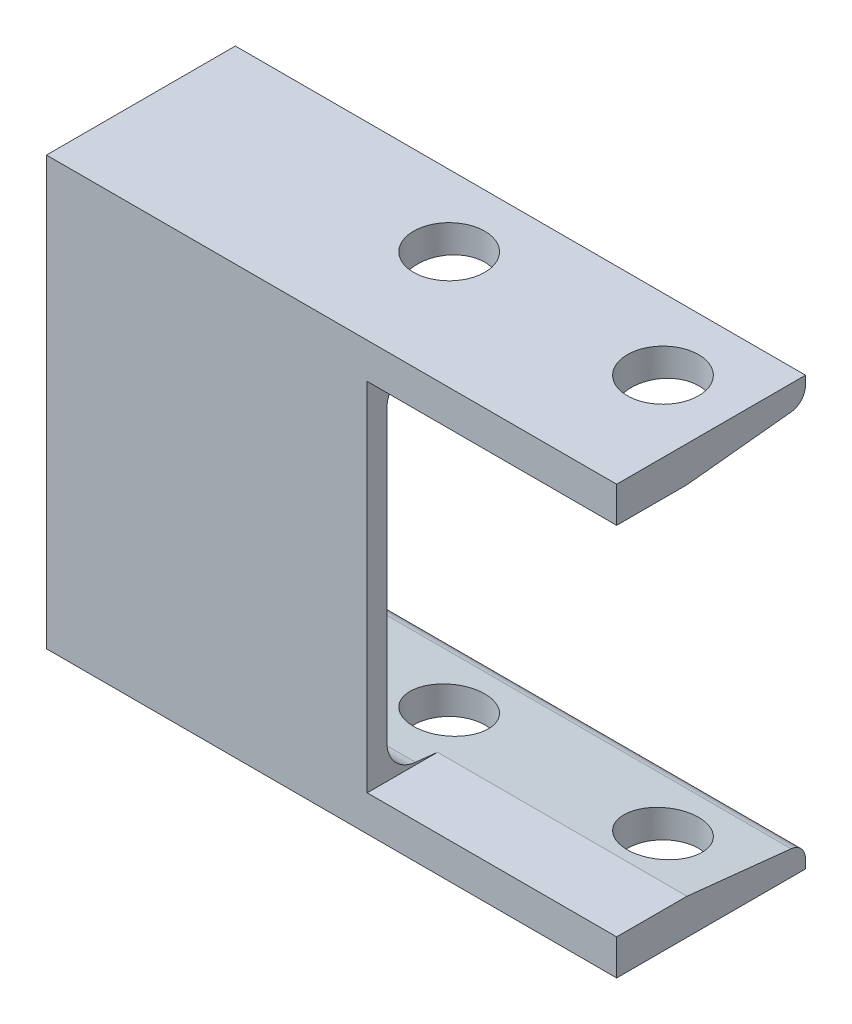
SolidWorks part; units mm, degrees
material "普通碳钢"
ref_plane "Front Plane" through (0, 0, 0) normal (0, 0, 1) x (1, 0, 0)
ref_plane "Top Plane" through (0, 0, 0) normal (0, 1, 0) x (1, 0, 0)
ref_plane "Right Plane" through (0, 0, 0) normal (1, 0, 0) x (0, 0, -1)
sketch3d "3DSketch1"
  line L0 (0, 0, 0) -> (160, 0, 0)
  dimension "D1" = 160
other "C-channel 12(1)"
ref_plane "Plane1" through (0, 0, 0) normal (1, 0, 0) x (0, 0, -1)
sketch "Sketch11" plane through (0, 0, 0) normal (1, 0, 0) x (0, 0, -1)
  line L0 (53, 120) -> (0, 120)
  line L1 (53, 0) -> (0, 0)
  line L2 (0, 120) -> (0, 0)
  line L3 (-9.5694, 60) -> (49.7414, 60) construction
  line L4 (5.5, 100.4001) -> (5.5, 19.5999)
  line L5 (53, 0) -> (53, 2.452)
  line L6 (53, 120) -> (53, 117.548)
  line L7 (13.5592, 10.6492) -> (48.9704, 6.9273)
  line L17 (13.5592, 109.3508) -> (48.9704, 113.0727)
  arc A0 (48.9704, 113.0727) -> (53, 117.548) centre (48.5, 117.548) ccw
  arc A1 (48.9704, 6.9273) -> (53, 2.452) centre (48.5, 2.452) cw
  arc A2 (5.5, 19.5999) -> (13.5592, 10.6492) centre (14.5, 19.5999) ccw
  arc A10 (5.5, 100.4001) -> (13.5592, 109.3508) centre (14.5, 100.4001) cw
  point P6 (0, 0)
  point P8 (0, 60)
  point P9 (5.5, 25.8841)
  point P10 (26.5, 120)
  point P13 (53, 113.4962)
  point P14 (29.25, 111)
  point P19 (5.5, 60)
sketch "Sketch2" plane through (0, 0, 0) normal (0, 0, 1) x (1, 0, 0)
  line L0 (190, 60) -> (160, 60) construction
  line L1 (90, 110) -> (190, 110)
  line L2 (90, 110) -> (90, 10)
  line L3 (90, 10) -> (190, 10)
  line L4 (190, 110) -> (190, 10)
  line L5 (160, 120) -> (160, 0) construction
  line L6 (0, 120) -> (0, 0) construction
  dimension "D1" = 100
  dimension "D2" = 90
  dimension "D3" = 100
extrude "Cut-Extrude1" cut sketch "Sketch2" against normal blind 40
sketch "Sketch3" plane through (0, 0, 0) normal (0, -1, 0) x (1, 0, 0)
  line L0 (0, -33) -> (160, -33) construction
  line L1 (0, 0) -> (0, -53) construction
  line L2 (160, 0) -> (160, -53) construction
  line L3 (0, 0) -> (160, 0) construction
  circle A0 centre (140, -33) radius 10
  circle A1 centre (80, -33) radius 10
  dimension "D1" = 20
  dimension "D2" = 20
  dimension "D3" = 33
  dimension "D4" = 80
  dimension "D5" = 60
extrude "Cut-Extrude2" cut sketch "Sketch3" against normal up to surface (120 mm away) up to face at (80, 120, -26.5)
equation "\"RI@Sketch11\" = \"D1@Sketch11\""
equation "\"D3@Sketch11\" =  ( \"BF@Sketch11\" - \"D6@Sketch11\" )  / 2"
